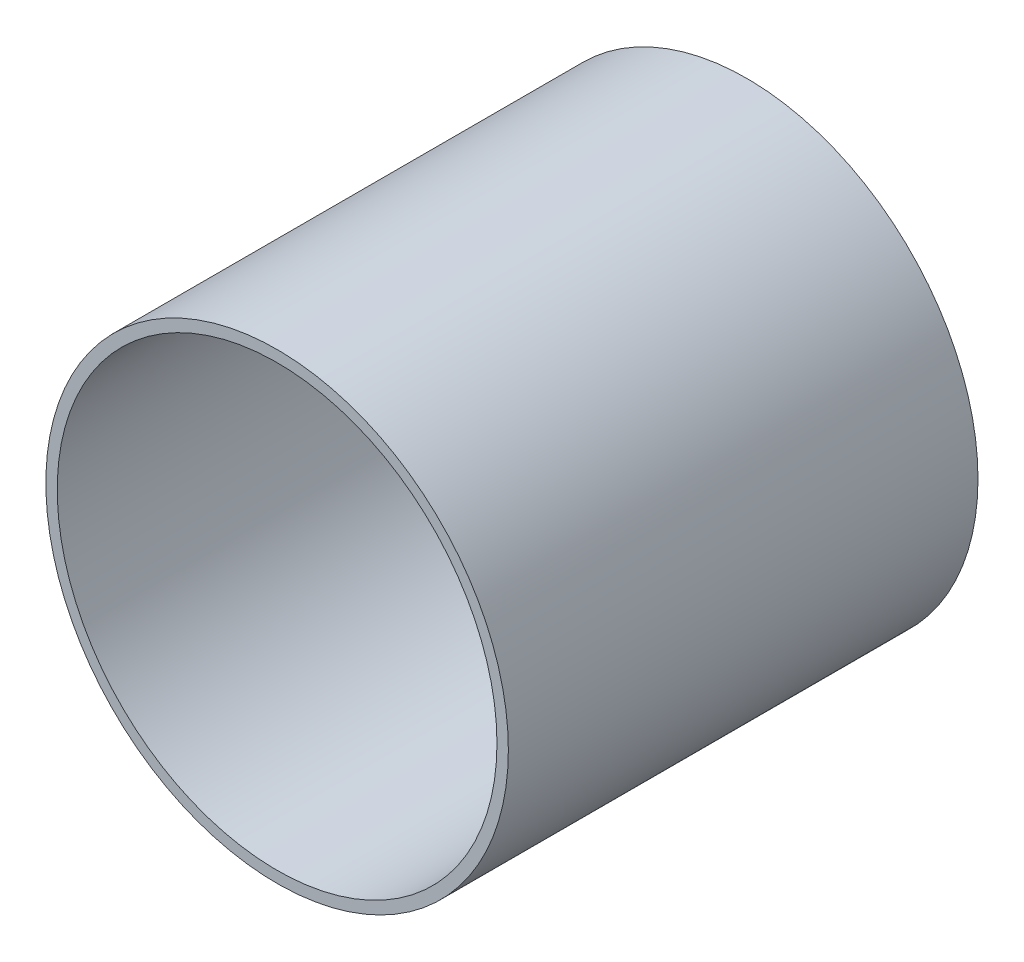
SolidWorks part; units mm, degrees
ref_plane "Front Plane" through (0, 0, 0) normal (0, 0, 1) x (1, 0, 0)
ref_plane "Top Plane" through (0, 0, 0) normal (0, 1, 0) x (1, 0, 0)
ref_plane "Right Plane" through (0, 0, 0) normal (1, 0, 0) x (0, 0, -1)
sketch "Sketch1" plane through (0, 0, 0) normal (0, 0, 1) x (1, 0, 0)
  circle A0 centre (0, 0) radius 162.5
  circle A1 centre (0, 0) radius 154.5
  dimension "D1" = 325
  dimension "D2" = 8
extrude "Boss-Extrude1" add sketch "Sketch1" along normal blind 330
